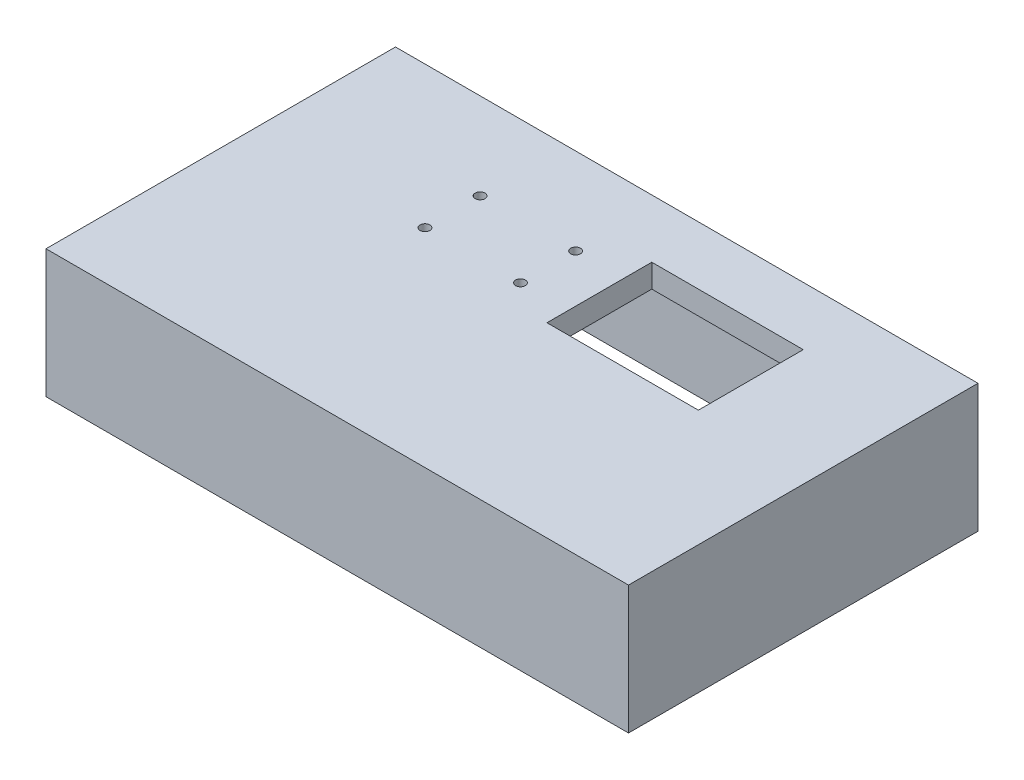
SolidWorks part; units mm, degrees
ref_plane "前视基准面" through (0, 0, 0) normal (0, 0, 1) x (1, 0, 0)
ref_plane "上视基准面" through (0, 0, 0) normal (0, 1, 0) x (1, 0, 0)
ref_plane "右视基准面" through (0, 0, 0) normal (1, 0, 0) x (0, 0, -1)
sketch "草图1" plane through (0, 0, 0) normal (0, 0, 1) x (1, 0, 0)
  line L1 (-157.4817, 68.4474) -> (92.5183, 68.4474)
  line L2 (-157.4817, 68.4474) -> (-157.4817, 13.4474)
  line L3 (-157.4817, 13.4474) -> (92.5183, 13.4474)
  line L4 (92.5183, 68.4474) -> (92.5183, 13.4474)
  dimension "D1" = 250
  dimension "D2" = 55
extrude "凸台-拉伸1" add sketch "草图1" along normal blind 150
sketch "草图2" plane through (0, 13.4474, 0) normal (0, -1, 0) x (1, 0, 0)
  line L4 (-147.4817, 140) -> (82.5183, 140)
  line L5 (82.5183, 140) -> (82.5183, 10)
  line L6 (82.5183, 10) -> (-147.4817, 10)
  line L9 (-157.4817, 150) -> (92.5183, 150) construction
  line L10 (92.5183, 150) -> (92.5183, 0) construction
  line L11 (-157.4817, 0) -> (92.5183, 0) construction
  line L12 (-147.4817, 140) -> (-147.4817, 10)
  line L13 (-157.4817, 150) -> (-157.4817, 0) construction
  dimension "D1" = 10
  dimension "D2" = 10
  dimension "D3" = 10
  dimension "D4" = 10
extrude "切除-拉伸1" cut sketch "草图2" against normal blind 45
sketch "草图4" plane through (0, 58.4474, 0) normal (0, -1, 0) x (1, 0, 0)
  line L0 (-157.4817, 0) -> (92.5183, 0) construction
  line L1 (-22.4817, 70) -> (42.5183, 70)
  line L2 (-22.4817, 70) -> (-22.4817, 25)
  line L3 (-22.4817, 25) -> (42.5183, 25)
  line L4 (42.5183, 70) -> (42.5183, 25)
  line L6 (92.5183, 150) -> (92.5183, 0) construction
  dimension "D1" = 25
  dimension "D2" = 50
  dimension "D3" = 65
  dimension "D4" = 45
extrude "切除-拉伸2" cut sketch "草图4" against normal through all
extrude "切除-拉伸8" cut sketch "草图10" against normal up to surface (17.7 mm away) up to face at (10.0183, 58.4474, 47.5)
sketch "草图10" plane through (971.2623, 76.1474, 1019.1439) normal (0, 1, 0) x (1, 0, 0)
  line L0 (-1055.2503, 985.1439) -> (-1055.2503, 955.1439) construction
  line L3 (-1014.2503, 985.1439) -> (-1014.2503, 955.1439) construction
  line L6 (-1060.2503, 981.9423) -> (-1009.2503, 981.9423) construction
  line L9 (-1060.2503, 958.2923) -> (-1009.2503, 958.2923) construction
  circle A0 centre (-1055.2503, 981.9423) radius 2.1
  circle A1 centre (-1055.2503, 958.2923) radius 2.1
  circle A2 centre (-1014.2503, 958.2923) radius 2.1
  circle A3 centre (-1014.2503, 981.9423) radius 2.1
